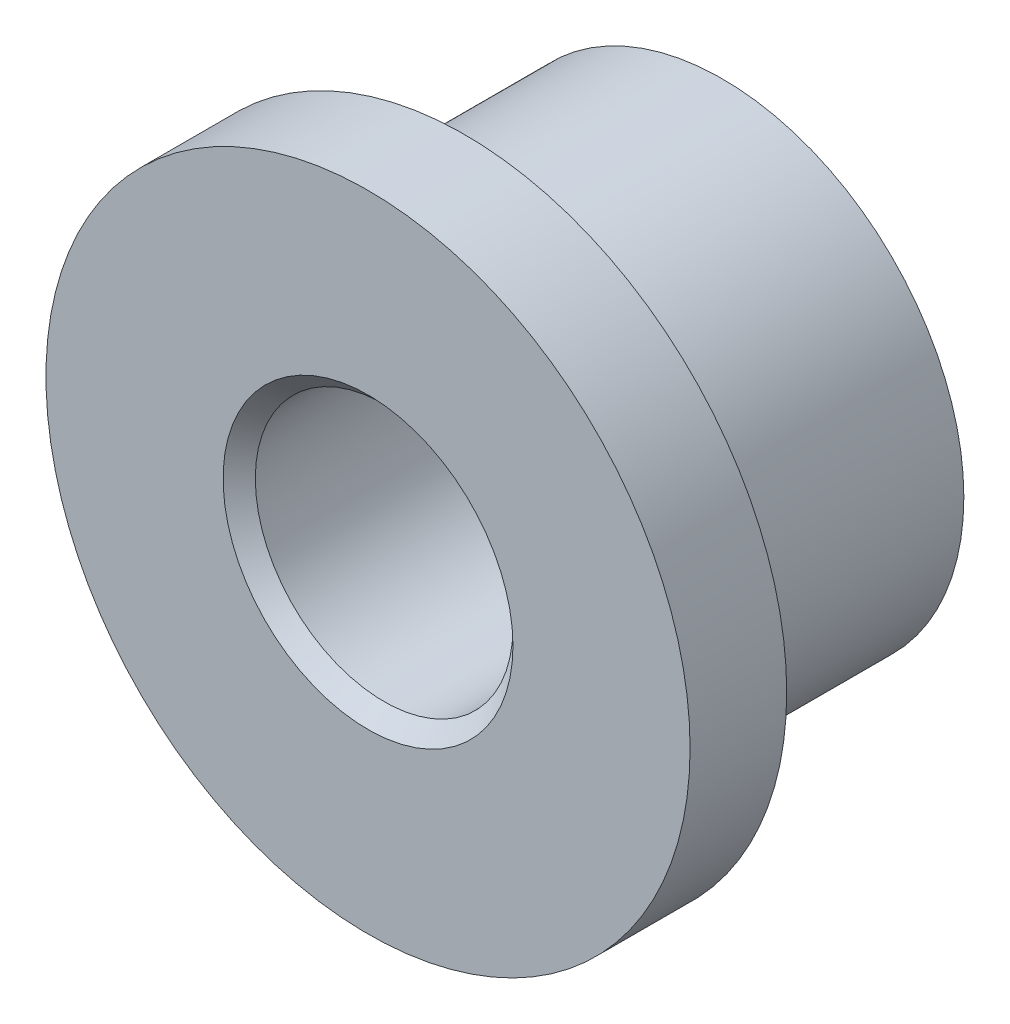
from build123d import *

# Parameters (mm, degrees)
SKETCH_1_R      = 7.5
SKETCH_1_R_2    = 4
EXTRUDE_1_DEPTH = 8
EXTRUDE_START   = 3
SKETCH_2_R      = 10
SKETCH_2_R_2    = 4
EXTRUDE_2_DEPTH = 3
CHAMFER_1_SIZE  = 0.5


with BuildPart() as part:
    # 草图1 → 凸台-拉伸1 (new body)
    with BuildSketch(Plane.XY):
        with Locations((145.504664302, 180.568940096)):
            Circle(SKETCH_1_R)
        with Locations((145.504664302, 180.568940096)):
            Circle(SKETCH_1_R_2, mode=Mode.SUBTRACT)
    extrude(amount=-EXTRUDE_1_DEPTH)

    # 草图2 → 凸台-拉伸2 (add)
    with BuildSketch(Plane.XY.offset(EXTRUDE_START)):
        with Locations((145.504664302, 180.568940096)):
            Circle(SKETCH_2_R)
        with Locations((145.504664302, 180.568940096)):
            Circle(SKETCH_2_R_2, mode=Mode.SUBTRACT)
    extrude(amount=-EXTRUDE_2_DEPTH)

    # 倒角1
    chamfer_1_edges = [part.edges().sort_by_distance(p)[0] for p in [
        (141.504664302, 180.568940096, 3),
        (141.504664302, 180.568940096, -8),
    ]]
    chamfer(chamfer_1_edges, length=CHAMFER_1_SIZE)


solid = part.part
